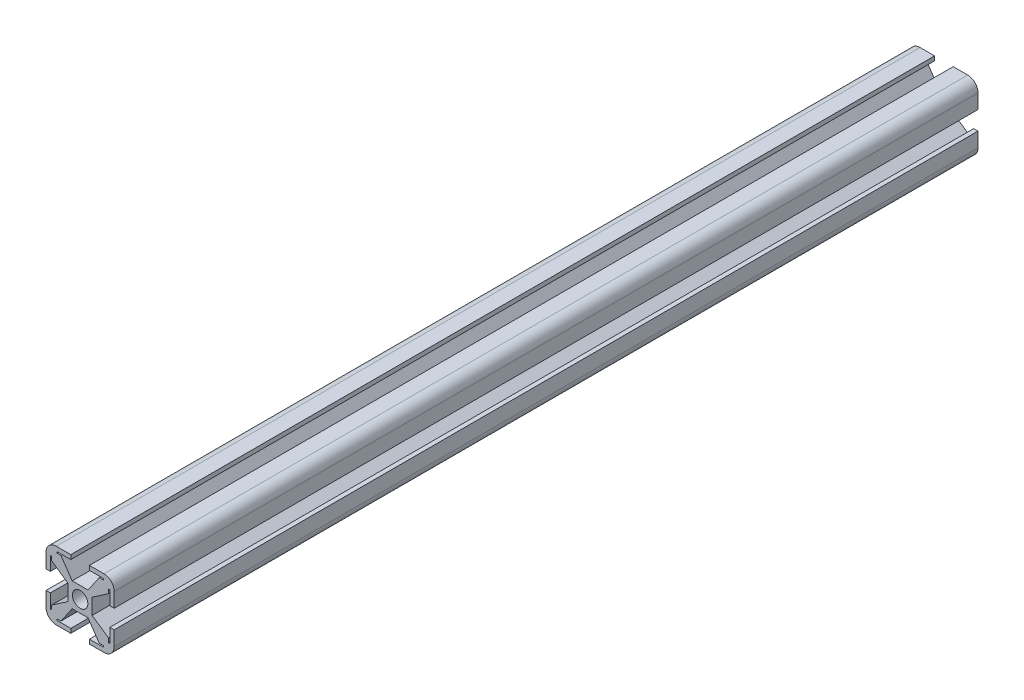
from build123d import *

# Parameters (mm, degrees)
SKETCH_1_W               = 30
SKETCH_1_H               = 30
EXTRUDE_1_DEPTH          = 190
FILLET_1_R               = 4.5
SKETCH_2_W               = 8.2
SKETCH_2_H               = 0.3
SKETCH_2_H_2             = 1.9
SKETCH_2_R               = 3.4
CUT_EXTRUDE_1_DEPTH      = 381.59164468
PATTERN_CIRCULAR_1_COUNT = 4


with BuildPart() as part:
    # 草图1 → 凸台-拉伸1 (new, symmetric)
    with BuildSketch(Plane.XY):
        Rectangle(SKETCH_1_W, SKETCH_1_H)
    extrude(amount=EXTRUDE_1_DEPTH, both=True)

    # 圆角1
    fillet_1_edges = [part.edges().sort_by_distance(p)[0] for p in [
        (-15, 15, 0),
        (15, 15, 0),
        (15, -15, 0),
        (-15, -15, 0),
    ]]
    fillet(fillet_1_edges, radius=FILLET_1_R)

    # 草图2 → 切除-拉伸1 (cut, through all)
    with BuildSketch(Plane.XY.offset(190)):
        with Locations((0, 12.95)):
            Rectangle(SKETCH_2_W, SKETCH_2_H)
        with Locations((0, 14.05)):
            Rectangle(SKETCH_2_W, SKETCH_2_H_2)
        Polygon((10.25, 13.1), (4.1, 13.1), (4.1, 12.8), (-4.1, 12.8), (-4.1, 13.1), (-10.25, 13.1), (-10.25, 12.5), (-8.429704265, 12.5), (8.429704265, 12.5), (10.25, 12.5), align=None)
        Polygon((3.479704265, 5.3), (8.429704265, 12.5), (-8.429704265, 12.5), (-3.479704265, 5.3), align=None)
        Circle(SKETCH_2_R)
    cut_extrude_1 = extrude(amount=-CUT_EXTRUDE_1_DEPTH, mode=Mode.SUBTRACT)

    # 阵列(圆周)1: 切除-拉伸1 ×4 about axis
    pattern_circular_1_axis = Axis((0, 0, 0), (0, 0, 1))
    for i in range(1, PATTERN_CIRCULAR_1_COUNT):
        add(cut_extrude_1.rotate(pattern_circular_1_axis, i * 360 / PATTERN_CIRCULAR_1_COUNT), mode=Mode.SUBTRACT)


solid = part.part
